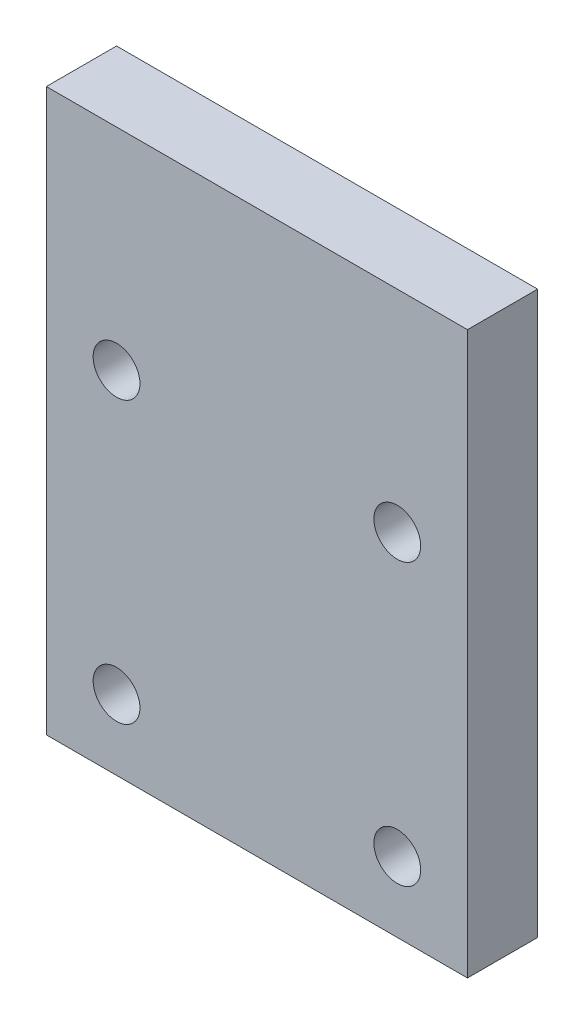
from build123d import *

# Parameters (mm, degrees)
SKETCH1_W                 = 150
SKETCH1_H                 = 200
BOSS_EXTRUDE1_DEPTH       = 25
F_3_4_10_THREADED_HOLE1_D = 16.66748


with BuildPart() as part:
    # Sketch1 → Boss-Extrude1 (new body)
    with BuildSketch(Plane.XY):
        with Locations((75, 100)):
            Rectangle(SKETCH1_W, SKETCH1_H)
    extrude(amount=BOSS_EXTRUDE1_DEPTH)

    # 3/4-10 Threaded hole1 (through all)
    with Locations(Plane(origin=(25, 125, 25), x_dir=(1, 0, 0), z_dir=(0, 0, 1))):
        with Locations((0, 0), (100, 0), (0, -100), (100, -100)):
            Hole(F_3_4_10_THREADED_HOLE1_D / 2)


solid = part.part
